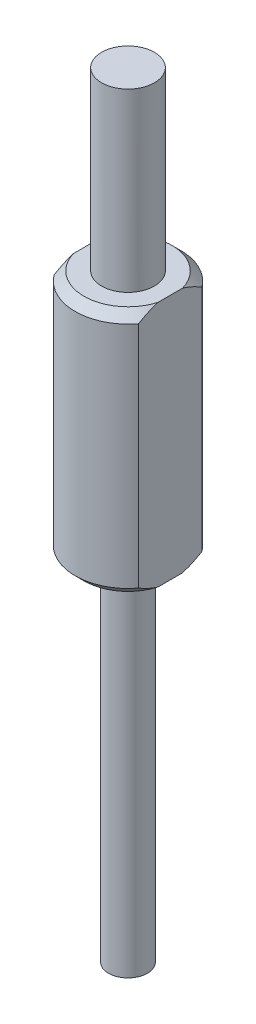
from build123d import *

# Parameters (mm, degrees)
SKETCH_1_R          = 1.5
EXTRUDE_1_DEPTH     = 10
SKETCH_2_R          = 3
M6X0_75P_DEPTH      = 14
SKETCH_3_R          = 1.1
EXTRUDE_3_DEPTH     = 20
CHAMFER_1_SIZE      = 0.5
SKETCH_4_W          = 2.061421144
SKETCH_4_H          = 7.488665512
CUT_EXTRUDE_1_DEPTH = 45.204072211


with BuildPart() as part:
    # 草图1 → 凸台-拉伸1 (new body)
    with BuildSketch(Plane(origin=(0, 0, 0), x_dir=(1, 0, 0), z_dir=(0, 1, 0))):
        with Locations(Location((0, 0, 0), (0, 0, 270))):
            Circle(SKETCH_1_R)
    extrude(amount=EXTRUDE_1_DEPTH)

    # 草图2 → M6X0.75P (add)
    with BuildSketch(Plane.XZ):
        with Locations(Location((0, 0, 0), (0, 0, 270))):
            Circle(SKETCH_2_R)
    extrude(amount=M6X0_75P_DEPTH)

    # 草图3 → 凸台-拉伸3 (add)
    with BuildSketch(Plane.XZ.offset(14)):
        with Locations(Location((0, 0, 0), (0, 0, 270))):
            Circle(SKETCH_3_R)
    extrude(amount=EXTRUDE_3_DEPTH)

    # 倒角1
    chamfer_1_edges = [part.edges().sort_by_distance(p)[0] for p in [
        (0, 0, 3),
        (0, -14, 3),
    ]]
    chamfer(chamfer_1_edges, length=CHAMFER_1_SIZE)

    # 草图4 → 切除-拉伸1 (cut, through all)
    with BuildSketch(Plane(origin=(0, 10, 0), x_dir=(1, 0, 0), z_dir=(0, 1, 0))):
        with Locations((3.430710572, 0.052409012)):
            Rectangle(SKETCH_4_W, SKETCH_4_H)
    cut_extrude_1 = extrude(amount=-CUT_EXTRUDE_1_DEPTH, mode=Mode.SUBTRACT)

    # 镜向1: 切除-拉伸1 across plane
    add(cut_extrude_1.mirror(Plane(origin=(0, 0, 0), x_dir=(0, 0, 1), z_dir=(1, 0, 0))), mode=Mode.SUBTRACT)


solid = part.part
